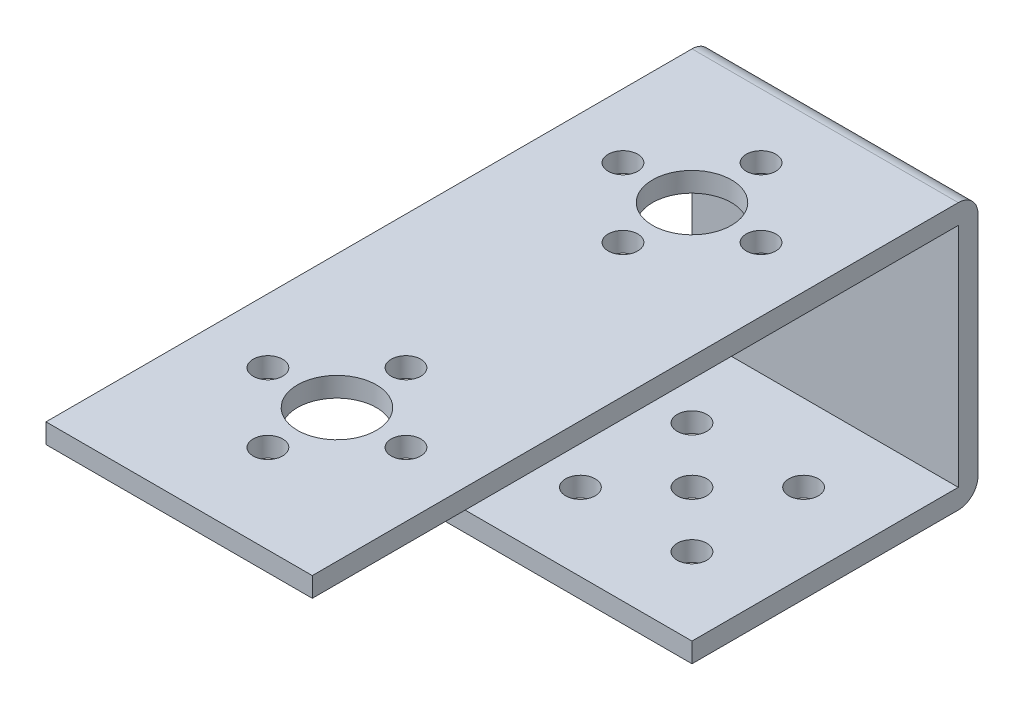
SolidWorks part; units mm, degrees
ref_plane "Front Plane" through (0, 0, 0) normal (0, 0, 1) x (1, 0, 0)
ref_plane "Top Plane" through (0, 0, 0) normal (0, 1, 0) x (1, 0, 0)
ref_plane "Right Plane" through (0, 0, 0) normal (1, 0, 0) x (0, 0, -1)
other "Configuration Table"
sketch "Sketch1" plane through (0, 0, 0) normal (0, 0, 1) x (1, 0, 0)
  line L1 (-13.5, 13.5) -> (13.5, 13.5)
  line L2 (-13.5, 13.5) -> (-13.5, -13.5)
  line L3 (-13.5, -13.5) -> (13.5, -13.5)
  line L4 (13.5, 13.5) -> (13.5, -13.5)
  line L5 (-13.5, 13.5) -> (13.5, -13.5) construction
  line L6 (-13.5, -13.5) -> (13.5, 13.5) construction
  point P0 (0, 0)
  dimension "D1" = 27
  dimension "27" = 27
extrude "Boss-Extrude1" add sketch "Sketch1" along normal blind 29
sketch "Sketch2" plane through (13.5, 0, 0) normal (1, 0, 0) x (0, 0, -1)
  line L0 (-29, -13.5) -> (-29, 13.5) construction
  line L1 (-29, 11.5) -> (-2, 11.5)
  line L2 (-29, 11.5) -> (-29, -11.5)
  line L3 (-29, -11.5) -> (-2, -11.5)
  line L4 (-2, 11.5) -> (-2, -11.5)
  line L5 (-29, 13.5) -> (0, 13.5) construction
  line L6 (-29, -13.5) -> (0, -13.5) construction
  line L7 (0, -13.5) -> (0, 13.5) construction
  dimension "D1" = 2
  dimension "D2" = 2
  dimension "D3" = 2
extrude "Cut-Extrude1" cut sketch "Sketch2" against normal blind 27
sketch "Sketch4" plane through (0, 13.5, 0) normal (0, 1, 0) x (1, 0, 0)
  line L0 (0, 0) -> (0, -30.566) construction
  line L2 (13.5, -29) -> (-13.5, -29) construction
  line L3 (0, -15.5) -> (28.6851, -15.5) construction
  circle A0 centre (0, -15.5) radius 4
  circle A1 centre (0, -15.5) radius 7 construction
  circle A2 centre (0, -8.5) radius 1.5
  circle A3 centre (7, -15.5) radius 1.5
  circle A4 centre (0, -22.5) radius 1.5
  circle A5 centre (-7, -15.5) radius 1.5
  point P19 (0, -15.5)
  dimension "D1" = 8
  dimension "D2" = 3
  dimension "D3" = 14
  dimension "D4" = 13.5
  dimension "D5" = 4
extrude "Cut-Extrude2" cut sketch "Sketch4" against normal up to next
sketch "Sketch5" plane through (0, -13.5, 0) normal (0, -1, 0) x (1, 0, 0)
  line L0 (0, 0) -> (0, 30.8311) construction
  line L1 (-13.5, 0) -> (13.5, 0) construction
  line L2 (-13.5, 29) -> (13.5, 29) construction
  line L3 (0, 15.5) -> (-10.8732, 26.3732) construction
  line L4 (0, 15.5) -> (11.3033, 26.8033) construction
  circle A0 centre (0, 15.5) radius 1.5
  circle A1 centre (0, 15.5) radius 8 construction
  circle A8 centre (-5.6569, 21.1569) radius 1.5
  circle A9 centre (5.6569, 21.1569) radius 1.5
  circle A10 centre (5.6569, 9.8431) radius 1.5
  circle A11 centre (-5.6569, 9.8431) radius 1.5
  point P20 (0, 15.5)
  point P27 (0, 15.5)
  dimension "D1" = 3
  dimension "D3" = 16
  dimension "D6" = 3
  dimension "D4" = 13.5
  dimension "D5" = 45
  dimension "D7" = 4
extrude "Cut-Extrude3" cut sketch "Sketch5" against normal up to next
fillet "Fillet1" radius 2 2 edges at (0, 13.5, 0) (0, -13.5, 0)
sketch "Sketch6" plane through (0, 0, 29) normal (0, 0, 1) x (1, 0, 0)
  line L4 (-13.5, 11.5) -> (13.5, 11.5)
  line L5 (13.5, 11.5) -> (13.5, 13.5)
  line L6 (13.5, 13.5) -> (-13.5, 13.5)
  line L7 (-13.5, 13.5) -> (-13.5, 11.5)
  line L8 (-13.5, 11.5) -> (13.5, 11.5)
  line L9 (13.5, 11.5) -> (13.5, 13.5)
  line L10 (13.5, 13.5) -> (-13.5, 13.5)
  line L11 (-13.5, 13.5) -> (-13.5, 11.5)
  dimension "D1" = 0
extrude "Boss-Extrude2" add sketch "Sketch6" along normal blind 38.5
sketch "Sketch7" plane through (0, 13.5, 0) normal (0, 1, 0) x (1, 0, 0)
  line L0 (0, 0) -> (0, -65.1809) construction
  line L1 (13.5, -67.5) -> (-13.5, -67.5) construction
  line L2 (0, -51.5) -> (-22.2306, -51.5) construction
  circle A0 centre (0, -51.5) radius 4
  circle A1 centre (0, -44.5) radius 1.5
  circle A2 centre (7, -51.5) radius 1.5
  circle A3 centre (0, -58.5) radius 1.5
  circle A4 centre (-7, -51.5) radius 1.5
  circle A6 centre (0, -51.5) radius 7 construction
  point P19 (0, -51.5)
  dimension "D1" = 8
  dimension "D2" = 3
  dimension "D3" = 14
  dimension "D4" = 16
  dimension "D5" = 4
extrude "Cut-Extrude4" cut sketch "Sketch7" against normal up to surface (2 mm away) up to face at (-1.5, 11.5, 8.5)
